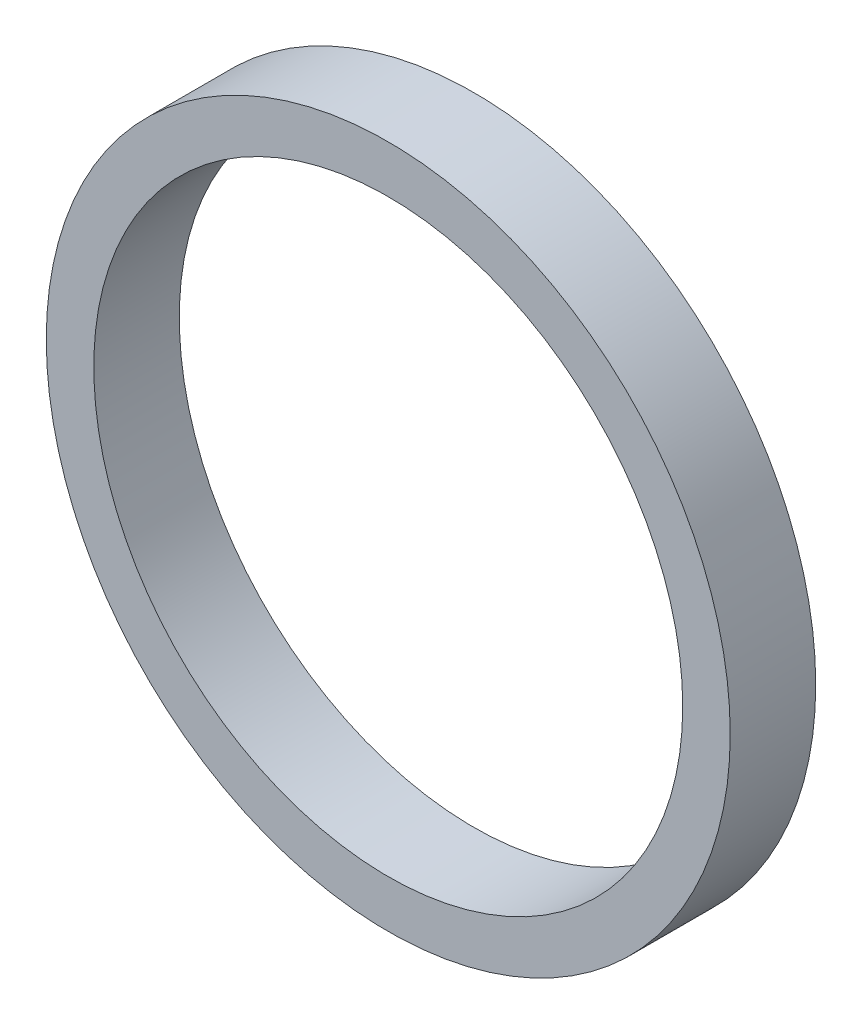
from build123d import *

# Parameters (mm, degrees)
SKETCH_1_R      = 18
SKETCH_1_R_2    = 15.5
EXTRUDE_1_DEPTH = 4.5


with BuildPart() as part:
    # 草图1 → 凸台-拉伸1 (new body)
    with BuildSketch(Plane.XY):
        Circle(SKETCH_1_R)
        Circle(SKETCH_1_R_2, mode=Mode.SUBTRACT)
    extrude(amount=EXTRUDE_1_DEPTH)


solid = part.part
